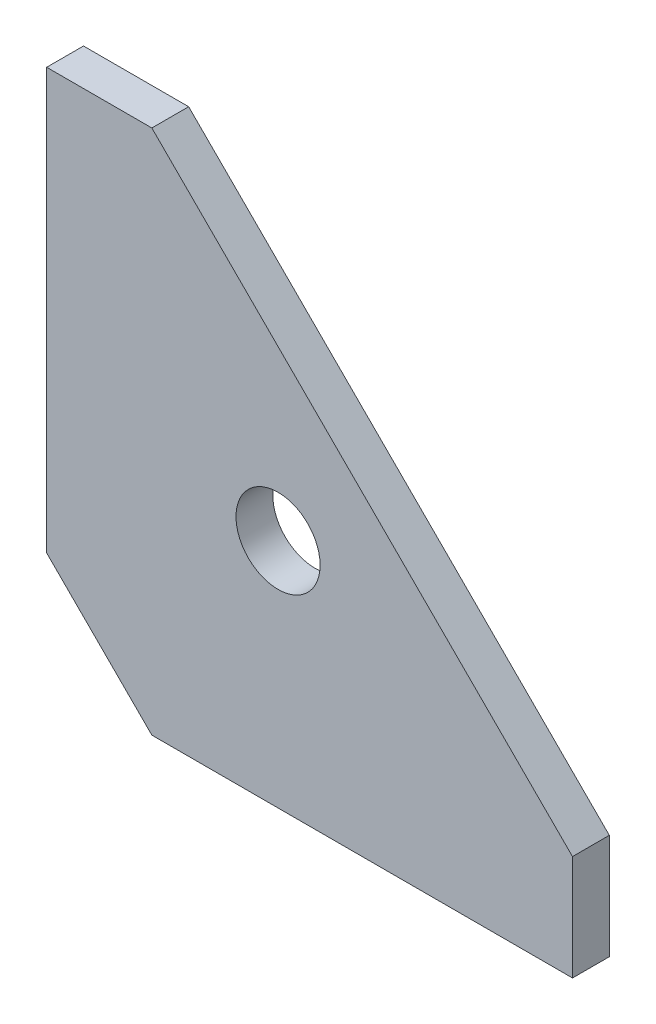
from build123d import *

# Parameters (mm, degrees)
SKETCH1_R           = 16
BOSS_EXTRUDE1_DEPTH = 14


with BuildPart() as part:
    # Sketch1 → Boss-Extrude1 (new body)
    with BuildSketch(Plane.XY):
        Polygon((0, 0), (40, 0), (200, -160), (200, -200), (40, -200), (0, -160), align=None)
        with Locations((88, -112)):
            Circle(SKETCH1_R, mode=Mode.SUBTRACT)
    extrude(amount=BOSS_EXTRUDE1_DEPTH)


solid = part.part
